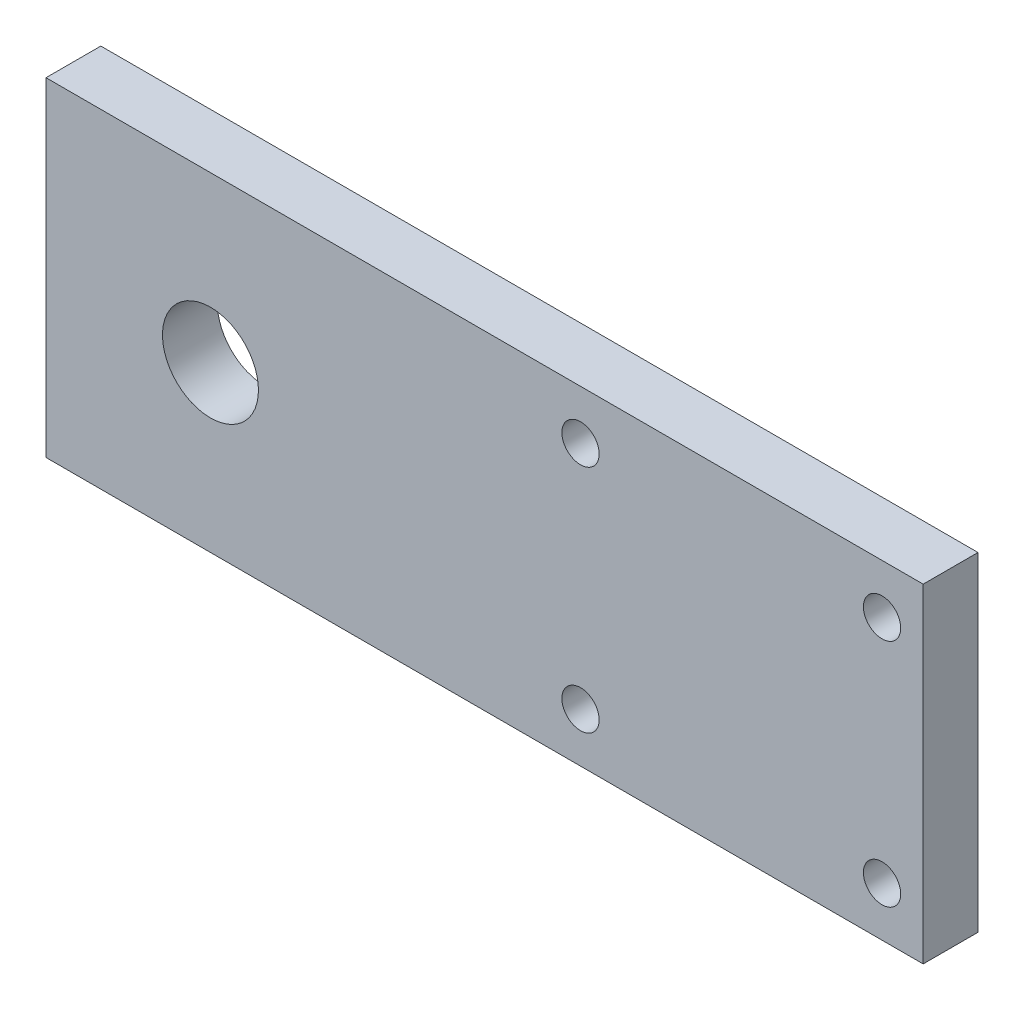
from build123d import *

# Parameters (mm, degrees)
SKETCH_1_W          = 160
SKETCH_1_H          = 60
EXTRUDE_1_DEPTH     = 10
HOLE_WIZARD_M20_1_D = 17.5
HOLE_WIZARD_M8_1_D  = 6.8


with BuildPart() as part:
    # 草图1 → 凸台-拉伸1 (new body)
    with BuildSketch(Plane.XY):
        Rectangle(SKETCH_1_W, SKETCH_1_H)
    extrude(amount=EXTRUDE_1_DEPTH)

    # M20 螺纹孔1 (through all)
    with Locations(Plane.XY.offset(10)):
        with Locations((-50, 0)):
            Hole(HOLE_WIZARD_M20_1_D / 2)

    # M8 螺纹孔1 (through all)
    with Locations(Plane.XY.offset(10)):
        with Locations((17.5, 21), (72.5, 21), (17.5, -21), (72.5, -21)):
            Hole(HOLE_WIZARD_M8_1_D / 2)


solid = part.part
